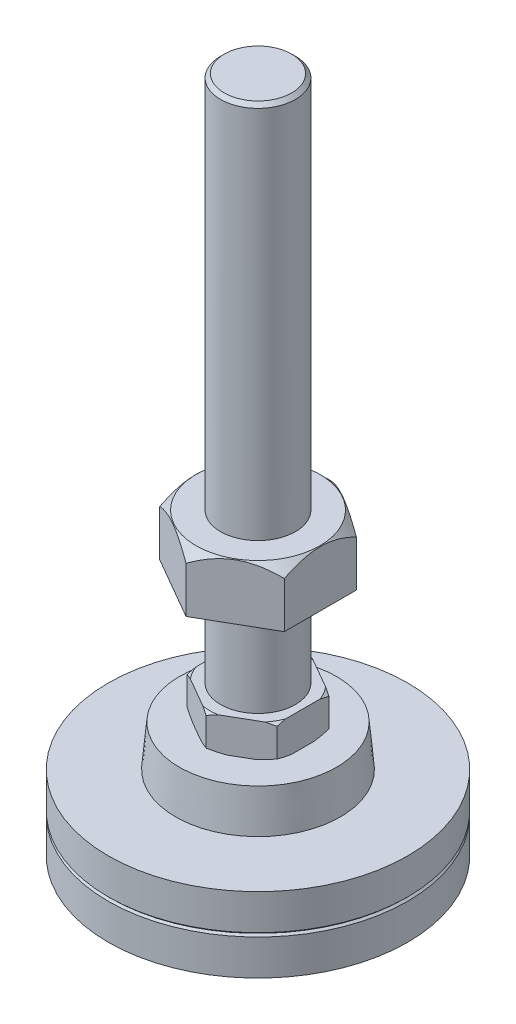
from build123d import *

# Parameters (mm, degrees)
BOSS_EXTRUDE1_DEPTH = 9
BOSS_EXTRUDE2_START = 39
SKETCH5_R           = 10
BOSS_EXTRUDE2_DEPTH = 15
CHAMFER1_SIZE       = 1


with BuildPart() as part:
    # Sketch1 → Revolve1 (revolve)
    with BuildSketch(Plane.XY, mode=Mode.PRIVATE) as revolve1_sk:
        Polygon((15, 0), (40, 0), (40, 9.5), (39.5, 10), (40, 10.5), (40, 20), (22, 20), (21, 31), (10, 31), (10, 181), (0, 181), (0, 15), (14, 15), align=None)
    revolve(revolve1_sk.sketch.rotate(Axis((0, 181, 0), (0, -1, 0)), 180), axis=Axis((0, 181, 0), (0, -1, 0)))

    # Sketch2 → Boss-Extrude1 (add)
    with BuildSketch(Plane(origin=(0, 31, 0), x_dir=(1, 0, 0), z_dir=(0, 1, 0))):
        Polygon((12, 6.92820323), (0, 13.856406461), (-12, 6.92820323), (-12, -6.92820323), (0, -13.856406461), (12, -6.92820323), align=None)
    extrude(amount=BOSS_EXTRUDE1_DEPTH)

    # Sketch3 → Cut-Revolve1 (revolve, cut)
    with BuildSketch(Plane(origin=(0, 0, 0), x_dir=(0, 0, -1), z_dir=(1, 0, 0))):
        Polygon((12.356406461, 31), (13.856406461, 31.866025404), (13.856406461, 31), align=None)
        Polygon((13.856406461, 39.422649731), (12.856406461, 40), (13.856406461, 40), align=None)
    revolve(axis=Axis((0, 181, 0), (0, 1, 0)), mode=Mode.SUBTRACT)

    # Sketch5 → Boss-Extrude2 (add)
    with BuildSketch(Plane(origin=(0, 41, 0), x_dir=(-1, 0, 0), z_dir=(0, 1, 0)).offset(BOSS_EXTRUDE2_START)):
        Polygon((0, 19.225763964), (-16.65, 9.612881982), (-16.65, -9.612881982), (0, -19.225763964), (16.65, -9.612881982), (16.65, 9.612881982), align=None)
        with Locations(Location((0, 0, 0), (0, 0, 90))):
            Circle(SKETCH5_R, mode=Mode.SUBTRACT)
    extrude(amount=-BOSS_EXTRUDE2_DEPTH)

    # Sketch7 → Cut-Revolve3 (revolve, cut)
    with BuildSketch(Plane(origin=(0, 0, 0), x_dir=(0, 0, -1), z_dir=(1, 0, 0)), mode=Mode.PRIVATE) as cut_revolve3_sk:
        Polygon((16.525763964, 80), (19.225763964, 77.3), (19.225763964, 80), align=None)
        Polygon((16.525763964, 41), (19.225763964, 43.7), (19.225763964, 41), align=None)
    revolve(cut_revolve3_sk.sketch.rotate(Axis((0, 181, 0), (0, 1, 0)), 180), axis=Axis((0, 181, 0), (0, 1, 0)), mode=Mode.SUBTRACT)

    # Chamfer1
    chamfer1_edges = [part.edges().sort_by_distance(p)[0] for p in [
        (10, 181, 0),
    ]]
    chamfer(chamfer1_edges, length=CHAMFER1_SIZE)


solid = part.part
